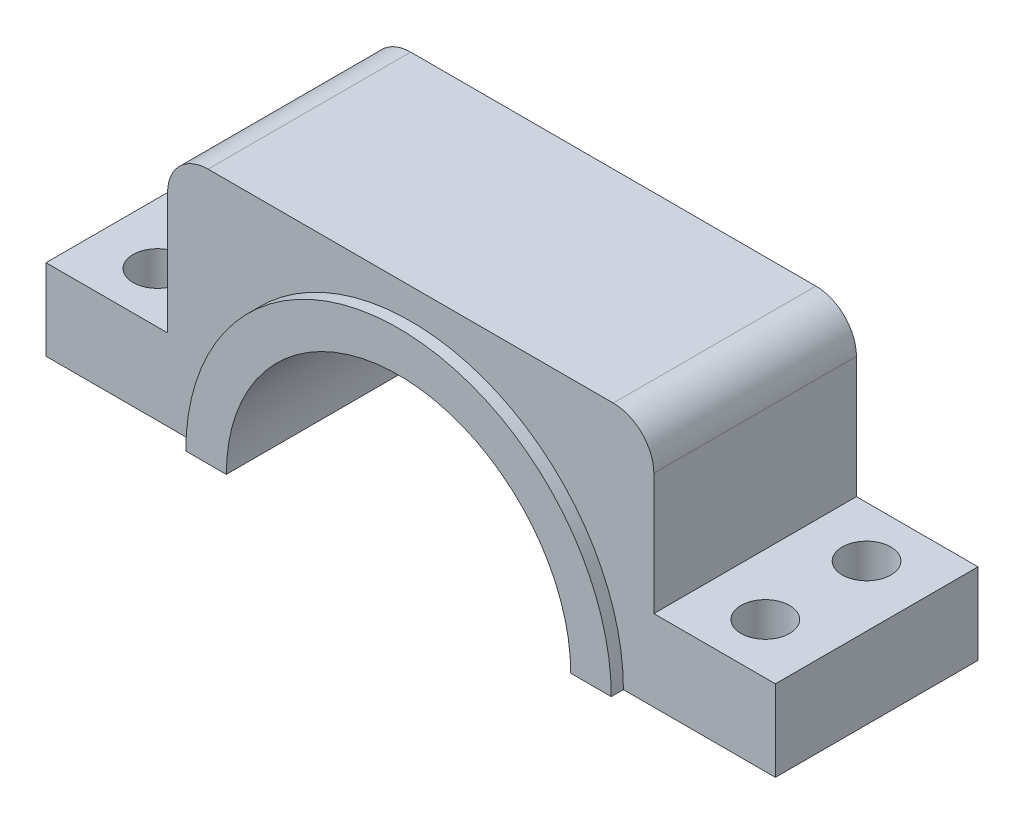
SolidWorks part; units mm, degrees
ref_plane "前视基准面" through (0, 0, 0) normal (0, 0, 1) x (1, 0, 0)
ref_plane "上视基准面" through (0, 0, 0) normal (0, 1, 0) x (1, 0, 0)
ref_plane "右视基准面" through (0, 0, 0) normal (1, 0, 0) x (0, 0, -1)
other "Configuration Table"
sketch "草图1" plane through (0, 0, 0) normal (0, 1, 0) x (1, 0, 0)
  line L1 (-60, -25) -> (60, -25)
  line L2 (-60, -25) -> (-60, 25)
  line L3 (-60, 25) -> (60, 25)
  line L4 (60, -25) -> (60, 25)
  line L5 (-60, -25) -> (60, 25) construction
  line L6 (-60, 25) -> (60, -25) construction
  point P0 (0, 0)
  dimension "D1" = 120
  dimension "D2" = 50
extrude "凸台-拉伸1" add sketch "草图1" along normal blind 60 contours L4 L3 L2 L1
sketch "草图2" plane through (0, 0, 25) normal (0, 0, 1) x (1, 0, 0)
  circle A0 centre (0, 0) radius 42.5
  dimension "D1" = 85
extrude "切除-拉伸1" cut sketch "草图2" against normal blind 60 contours A0
sketch "草图3" plane through (0, 0, 0) normal (0, -1, 0) x (1, 0, 0)
  line L0 (42.5, 25) -> (60, 25) construction
  line L1 (-90, -25) -> (-60, -25)
  line L2 (-90, -25) -> (-90, 25)
  line L3 (-90, 25) -> (-60, 25)
  line L4 (90, -25) -> (90, 25)
  line L5 (-90, -25) -> (90, 25) construction
  line L6 (-90, 25) -> (90, -25) construction
  line L7 (60, 25) -> (60, -25) construction
  line L8 (-60, 25) -> (-60, -25) construction
  line L9 (60, 25) -> (60, -25)
  line L10 (-60, 25) -> (-60, -25)
  line L11 (60, 25) -> (90, 25)
  line L12 (60, -25) -> (90, -25)
  point P0 (0, 0)
  dimension "D1" = 180
extrude "凸台-拉伸2" add sketch "草图3" against normal blind 20
fillet "圆角1" radius 10 2 edges at (60, 60, 0) (-60, 60, 0)
sketch "草图4" plane through (0, 0, 25) normal (0, 0, 1) x (1, 0, 0)
  line L0 (-52.5, 0) -> (-42.5, 0)
  line L3 (42.5, 0) -> (52.5, 0)
  arc A0 (52.5, 0) -> (-52.5, 0) centre (0, 0) ccw
  arc A1 (42.5, 0) -> (-42.5, 0) centre (0, 0) ccw construction
  arc A2 (42.5, 0) -> (-42.5, 0) centre (0, 0) ccw
  dimension "D1" = 105
extrude "凸台-拉伸3" add sketch "草图4" along normal blind 3
mirror "镜向1" about plane through (0, 0, 0) normal (0, 0, 1) of "凸台-拉伸3"
sketch "草图5" plane through (0, 20, 0) normal (0, 1, 0) x (1, 0, 0)
  line L0 (0, 0) -> (0, 39.9576) construction
  line L1 (90, -25) -> (60, -25) construction
  line L2 (60, 25) -> (90, 25) construction
  circle A0 centre (75, 12.5) radius 6
  circle A1 centre (75, -12.5) radius 6
  circle A2 centre (-75, -12.5) radius 6
  circle A3 centre (-75, 12.5) radius 6
  dimension "D1" = 12
  dimension "D2" = 75
  dimension "D3" = 12.5
  dimension "D4" = 12.5
extrude "切除-拉伸2" cut sketch "草图5" against normal blind 67
